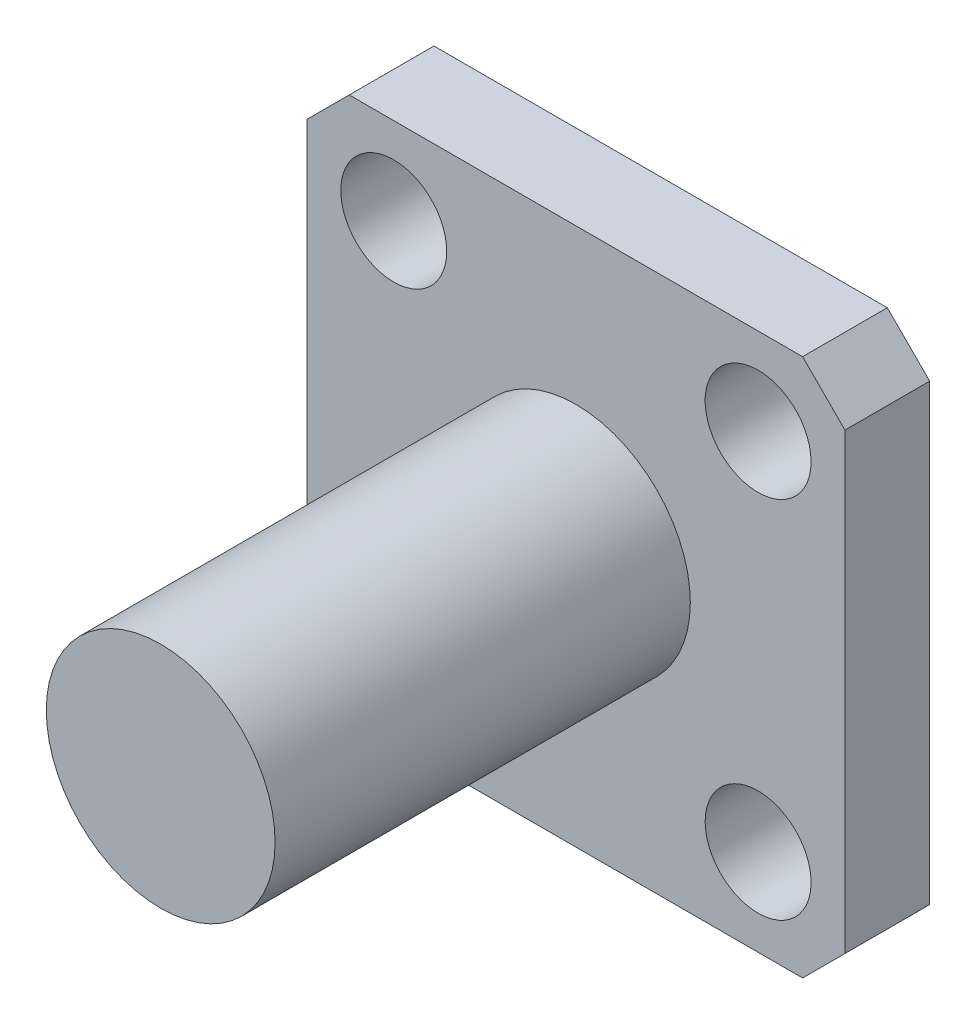
SolidWorks part; units mm, degrees
ref_plane "Front Plane" through (0, 0, 0) normal (0, 0, 1) x (1, 0, 0)
ref_plane "Top Plane" through (0, 0, 0) normal (0, 1, 0) x (1, 0, 0)
ref_plane "Right Plane" through (0, 0, 0) normal (1, 0, 0) x (0, 0, -1)
sketch "Sketch1" plane through (0, 0, 0) normal (0, 0, 1) x (1, 0, 0)
  line L0 (-12.7, -6.35) -> (0, -6.35) construction
  line L1 (0, 0) -> (-12.7, 0)
  line L2 (0, 0) -> (0, -12.7)
  line L3 (0, -12.7) -> (-12.7, -12.7)
  line L4 (-12.7, 0) -> (-12.7, -12.7)
  line L5 (0, -6.35) -> (-6.35, -6.35) construction
  line L6 (-6.35, -6.35) -> (-6.35, 0) construction
  circle A0 centre (-10.65, -2.05) radius 1.25
  circle A1 centre (-2.05, -2.05) radius 1.25
  circle A2 centre (-2.05, -10.65) radius 1.25
  circle A3 centre (-10.65, -10.65) radius 1.25
  dimension "D3" = 2.5
  dimension "D4" = 2.5
  dimension "D6" = 8.6
  dimension "D1" = 12.7
  dimension "D2" = 12.7
  dimension "D5" = 8.6
extrude "Boss-Extrude1" add sketch "Sketch1" along normal blind 2
chamfer "Chamfer1" distance 1 angle 45 4 edges at (-12.7, -12.7, 1) (0, -12.7, 1) (0, 0, 1) (-12.7, 0, 1)
sketch "Sketch2" plane through (0, 0, 2) normal (0, 0, 1) x (1, 0, 0)
  circle A0 centre (-6.35, -6.35) radius 2.7
  dimension "D1" = 5.4
extrude "Boss-Extrude2" add sketch "Sketch2" along normal blind 4.6
sketch "Sketch3" plane through (0, 0, 6.6) normal (0, 0, 1) x (1, 0, 0)
  circle A0 centre (-6.35, -6.35) radius 2.7
  dimension "D1" = 5.4
extrude "Boss-Extrude3" add sketch "Sketch3" along normal blind 5.2
